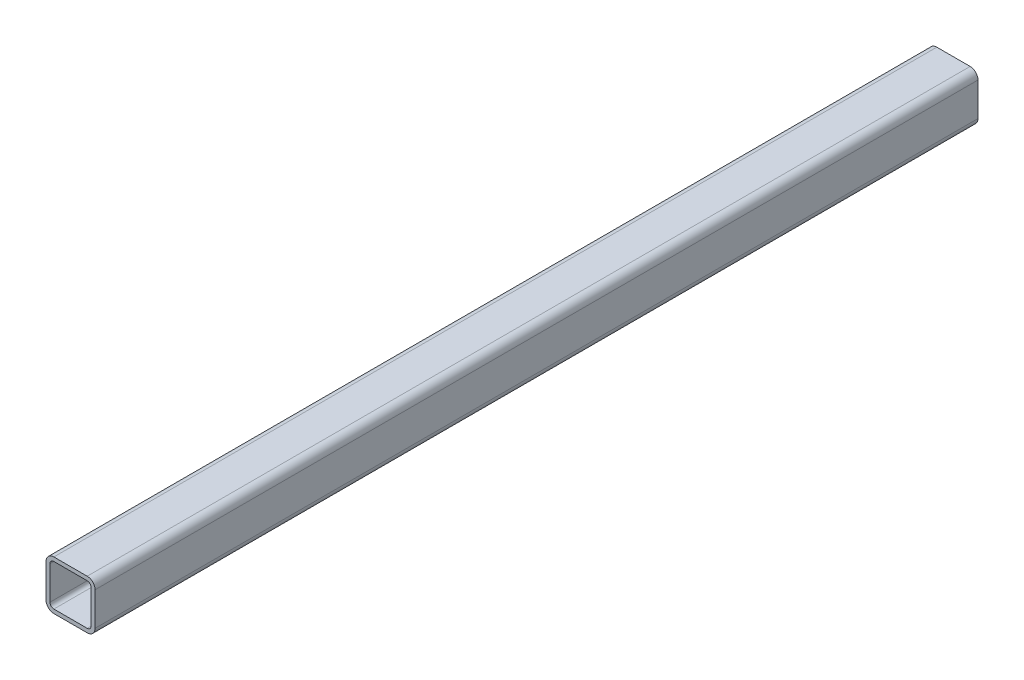
from build123d import *

# Parameters (mm, degrees)
BOSS_EXTRUDE1_DEPTH = 450


with BuildPart() as part:
    # Sketch1 → Boss-Extrude1 (new, symmetric)
    with BuildSketch(Plane.XY):
        with BuildLine():
            Line((-17, -25), (17, -25))
            ThreePointArc((17, -25), (22.656854249, -22.656854249), (25, -17))
            Line((25, -17), (25, 17))
            ThreePointArc((25, 17), (22.656854249, 22.656854249), (17, 25))
            Line((17, 25), (-17, 25))
            ThreePointArc((-17, 25), (-22.656854249, 22.656854249), (-25, 17))
            Line((-25, 17), (-25, -17))
            ThreePointArc((-25, -17), (-22.656854249, -22.656854249), (-17, -25))
        make_face()
        with BuildLine():
            Line((-17, 21), (17, 21))
            ThreePointArc((17, 21), (19.828427125, 19.828427125), (21, 17))
            Line((21, 17), (21, -17))
            ThreePointArc((21, -17), (19.828427125, -19.828427125), (17, -21))
            Line((17, -21), (-17, -21))
            ThreePointArc((-17, -21), (-19.828427125, -19.828427125), (-21, -17))
            Line((-21, -17), (-21, 17))
            ThreePointArc((-21, 17), (-19.828427125, 19.828427125), (-17, 21))
        make_face(mode=Mode.SUBTRACT)
    extrude(amount=BOSS_EXTRUDE1_DEPTH, both=True)


solid = part.part
